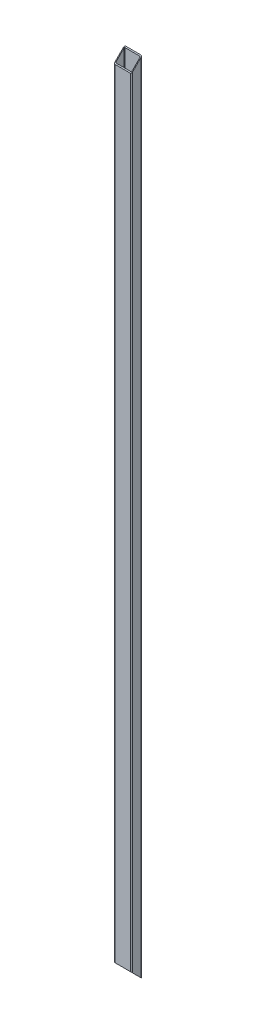
SolidWorks part; units mm, degrees
ref_plane "Front" through (0, 0, 0) normal (0, 0, 1) x (1, 0, 0)
ref_plane "Top" through (0, 0, 0) normal (0, 1, 0) x (1, 0, 0)
ref_plane "Right" through (0, 0, 0) normal (1, 0, 0) x (0, 0, -1)
sketch "Sketch1" plane through (0, 0, 0) normal (0, 1, 0) x (1, 0, 0)
  line L0 (-21.55, -12.7) -> (21.55, -12.7)
  line L1 (-21.55, -15) -> (21.55, -15)
  line L2 (-25, -11.55) -> (-25, 11.55)
  line L3 (-21.55, 15) -> (21.55, 15)
  line L4 (25, -11.55) -> (25, 11.55)
  line L5 (-25, -15) -> (25, 15) construction
  line L6 (-25, 15) -> (25, -15) construction
  line L7 (22.7, -11.55) -> (22.7, 11.55)
  line L8 (-21.55, 12.7) -> (21.55, 12.7)
  line L9 (-22.7, -11.55) -> (-22.7, 11.55)
  arc A0 (21.55, 15) -> (25, 11.55) centre (21.55, 11.55) cw
  arc A1 (-21.55, -15) -> (-25, -11.55) centre (-21.55, -11.55) cw
  arc A2 (21.55, -15) -> (25, -11.55) centre (21.55, -11.55) ccw
  arc A3 (-25, 11.55) -> (-21.55, 15) centre (-21.55, 11.55) cw
  arc A4 (21.55, -12.7) -> (22.7, -11.55) centre (21.55, -11.55) ccw
  arc A5 (21.55, 12.7) -> (22.7, 11.55) centre (21.55, 11.55) cw
  arc A6 (-22.7, 11.55) -> (-21.55, 12.7) centre (-21.55, 11.55) cw
  arc A7 (-21.55, -12.7) -> (-22.7, -11.55) centre (-21.55, -11.55) cw
  point P0 (0, 0)
  dimension "D3" = 3.45
  dimension "D1" = 50
  dimension "D2" = 30
  dimension "D4" = 2.3
extrude "Boss-Extrude1" add sketch "Sketch1" along normal blind 2270
sketch "Sketch2" plane through (25, 0, 0) normal (1, 0, 0) x (0, 0, -1)
  line L0 (15, 2270) -> (-15, 2240)
  line L1 (-15, 2270) -> (-15, 0) construction
  line L2 (-15, 2240) -> (-15, 2270)
  line L3 (-15, 2270) -> (15, 2270)
  line L4 (15, 0) -> (-15, 0)
  line L5 (-15, 0) -> (-15, 30)
  line L6 (-15, 30) -> (15, 0)
  dimension "D1" = 45
  dimension "D2" = 45
extrude "Cut-Extrude1" cut sketch "Sketch2" against normal through all both and the other way through all
